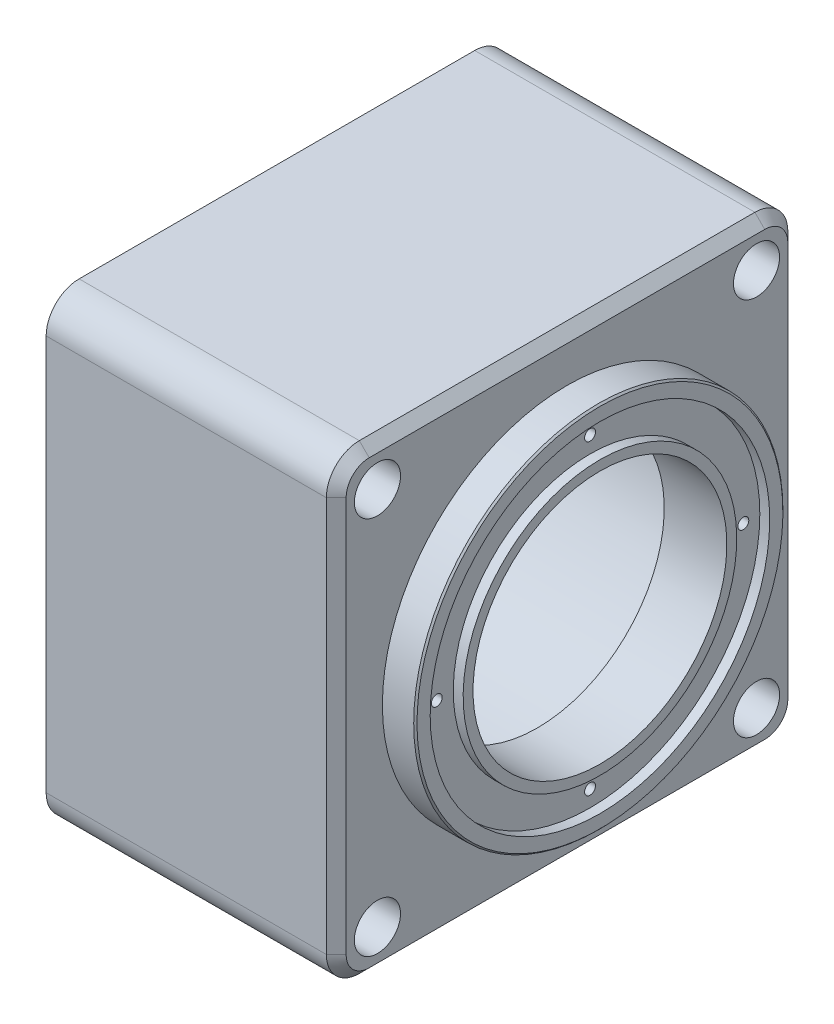
from build123d import *

# Parameters (mm, degrees)
SKETCH1_W               = 140
SKETCH1_H               = 140
BOSS_EXTRUDE1_DEPTH     = 88
SKETCH2_R               = 56
BOSS_EXTRUDE2_DEPTH     = 10
SKETCH3_R               = 60
CUT_EXTRUDE1_DEPTH      = 76
SKETCH4_R               = 38.5
CUT_EXTRUDE2_DEPTH      = 49
M10_TAPPED_HOLE1_D      = 8.5
M10_TAPPED_HOLE1_DEPTH  = 35
M10_TAPPED_HOLE1_TIP    = 2.553657631
M16_TAPPED_HOLE1_D      = 14
M16_TAPPED_HOLE1_DEPTH  = 35
M16_TAPPED_HOLE1_TIP    = 4.206024333
SKETCH14_R              = 55
CUT_EXTRUDE5_DEPTH      = 3
CHAMFER2_SIZE           = 0.5
BOSS_EXTRUDE3_START     = 44
SKETCH17_R              = 60
BOSS_EXTRUDE3_DEPTH     = 15
SKETCH18_R              = 55
CUT_EXTRUDE7_DEPTH      = 15
SKETCH22_R              = 60
CUT_EXTRUDE8_DEPTH      = 15
SKETCH23_R              = 51.5
SKETCH23_R_2            = 41.5
CUT_EXTRUDE9_DEPTH      = 3
CIRPATTERN1_COUNT       = 4
FILLET1_R               = 10
CHAMFER6_SIZE           = 3
SKETCH30_R              = 2.5
CUT_EXTRUDE12_DEPTH     = 12
G1_8_TAPPED_HOLE1_D     = 8.8
G1_8_TAPPED_HOLE1_DEPTH = 22.18
G1_8_TAPPED_HOLE1_TIP   = 2.643786724
SKETCH34_R              = 11
CUT_EXTRUDE14_DEPTH     = 3


with BuildPart() as part:
    # Sketch1 → Boss-Extrude1 (new body)
    with BuildSketch(Plane(origin=(0, 0, 0), x_dir=(0, -1, 0), z_dir=(1, 0, 0))):
        Rectangle(SKETCH1_W, SKETCH1_H)
    extrude(amount=BOSS_EXTRUDE1_DEPTH)

    # Sketch2 → Boss-Extrude2 (add)
    with BuildSketch(Plane(origin=(88, 0, 0), x_dir=(0, -1, 0), z_dir=(1, 0, 0))):
        with Locations(Location((0, 0, 0), (0, 0, 180))):
            Circle(SKETCH2_R)
    extrude(amount=BOSS_EXTRUDE2_DEPTH)

    # Sketch3 → Cut-Extrude1 (cut)
    with BuildSketch(Plane(origin=(0, 0, 0), x_dir=(0, -1, 0), z_dir=(-1, 0, 0))):
        Circle(SKETCH3_R)
    extrude(amount=-CUT_EXTRUDE1_DEPTH, mode=Mode.SUBTRACT)

    # Sketch4 → Cut-Extrude2 (cut)
    with BuildSketch(Plane(origin=(98, 0, 0), x_dir=(0, -1, 0), z_dir=(1, 0, 0))):
        with Locations(Location((0, 0, 0), (0, 0, 180))):
            Circle(SKETCH4_R)
    extrude(amount=-CUT_EXTRUDE2_DEPTH, mode=Mode.SUBTRACT)

    # M10 Tapped Hole1
    with Locations(Plane(origin=(0, 0, 0), x_dir=(0, 1, 0), z_dir=(-1, 0, 0))):
        with Locations((-35, 60), (35, 60), (60, 35), (60, -35), (35, -60), (-35, -60), (-60, -35), (-60, 35)):
            Hole(M10_TAPPED_HOLE1_D / 2, depth=M10_TAPPED_HOLE1_DEPTH)
            with Locations((0, 0, -(M10_TAPPED_HOLE1_DEPTH + M10_TAPPED_HOLE1_TIP / 2))):  # 118° drill point
                Cone(0, M10_TAPPED_HOLE1_D / 2, M10_TAPPED_HOLE1_TIP, mode=Mode.SUBTRACT)

    # M16 Tapped Hole1
    with Locations(Plane(origin=(88, 0, 0), x_dir=(0, -1, 0), z_dir=(1, 0, 0))):
        with Locations((57.5, 57.5), (-57.5, 57.5), (-57.5, -57.5), (57.5, -57.5)):
            Hole(M16_TAPPED_HOLE1_D / 2, depth=M16_TAPPED_HOLE1_DEPTH)
            with Locations((0, 0, -(M16_TAPPED_HOLE1_DEPTH + M16_TAPPED_HOLE1_TIP / 2))):  # 118° drill point
                Cone(0, M16_TAPPED_HOLE1_D / 2, M16_TAPPED_HOLE1_TIP, mode=Mode.SUBTRACT)

    # Sketch14 → Cut-Extrude5 (cut)
    with BuildSketch(Plane(origin=(76, 0, 0), x_dir=(0, -1, 0), z_dir=(-1, 0, 0))):
        Circle(SKETCH14_R)
    extrude(amount=-CUT_EXTRUDE5_DEPTH, mode=Mode.SUBTRACT)

    # Chamfer2
    chamfer2_edges = [part.edges().sort_by_distance(p)[0] for p in [
        (98, -56, 0),
    ]]
    chamfer(chamfer2_edges, length=CHAMFER2_SIZE)

    # Sketch17 → Boss-Extrude3 (add)
    with BuildSketch(Plane.ZY.offset(-76).offset(BOSS_EXTRUDE3_START)):
        with Locations(Location((0, 0, 0), (0, 0, 270))):
            Circle(SKETCH17_R)
    extrude(amount=-BOSS_EXTRUDE3_DEPTH)

    # Sketch18 → Cut-Extrude7 (cut)
    with BuildSketch(Plane.ZY.offset(-32)):
        with Locations(Location((0, 0, 0), (0, 0, 270))):
            Circle(SKETCH18_R)
    extrude(amount=-CUT_EXTRUDE7_DEPTH, mode=Mode.SUBTRACT)

    # Sketch22 → Cut-Extrude8 (cut)
    with BuildSketch(Plane.ZY.offset(-32)):
        with Locations(Location((0, 0, 0), (0, 0, 270))):
            Circle(SKETCH22_R)
    extrude(amount=-CUT_EXTRUDE8_DEPTH, mode=Mode.SUBTRACT)

    # Sketch23 → Cut-Extrude9 (cut)
    with BuildSketch(Plane(origin=(98, 0, 0), x_dir=(0, 0, -1), z_dir=(1, 0, 0))):
        with Locations(Location((0, 0, 0), (0, 0, 90))):
            Circle(SKETCH23_R)
        with Locations(Location((0, 0, 0), (0, 0, 90))):
            Circle(SKETCH23_R_2, mode=Mode.SUBTRACT)
    extrude(amount=-CUT_EXTRUDE9_DEPTH, mode=Mode.SUBTRACT)

    # Sketch25 → M4 Tapped Hole2 (revolve, cut)
    with BuildSketch(Plane(origin=(95, 46.5, 0), x_dir=(0, 0, -1), z_dir=(0, 1, 0))):
        Polygon((0, 0), (0, 11.091420021), (1.65, 10.1), (1.65, 0), align=None)
    m4_tapped_hole2 = revolve(axis=Axis((101.35, 46.5, 0), (-1, 0, 0)), mode=Mode.SUBTRACT)

    # CirPattern1: M4 Tapped Hole2 ×4 about axis
    cirpattern1_axis = Axis((0, 0, 0), (1, 0, 0))
    for i in range(1, CIRPATTERN1_COUNT):
        add(m4_tapped_hole2.rotate(cirpattern1_axis, i * 360 / CIRPATTERN1_COUNT), mode=Mode.SUBTRACT)

    # Fillet1
    fillet1_edges = [part.edges().sort_by_distance(p)[0] for p in [
        (44, -70, 70),
        (44, 70, 70),
        (44, 70, -70),
        (44, -70, -70),
    ]]
    fillet(fillet1_edges, radius=FILLET1_R)

    # Chamfer6
    chamfer6_edges = [part.edges().sort_by_distance(p)[0] for p in [
        (88, 0, -70),
        (88, -70, 0),
        (88, 70, 0),
        (88, 0, 70),
        (88, 67.071067812, 67.071067812),
        (88, 67.071067812, -67.071067812),
        (88, -67.071067812, 67.071067812),
        (88, -67.071067812, -67.071067812),
    ]]
    chamfer(chamfer6_edges, length=CHAMFER6_SIZE)

    # Sketch30 → Cut-Extrude12 (cut)
    with BuildSketch(Plane.XZ.offset(70)):
        with Locations(Location((43, 0, 0), (0, 0, 270))):
            Circle(SKETCH30_R)
    extrude(amount=-CUT_EXTRUDE12_DEPTH, mode=Mode.SUBTRACT)

    # G1/8 Tapped Hole1
    with Locations(Plane(origin=(0, -70, 0), x_dir=(-1, 0, 0), z_dir=(0, -1, 0))):
        with Locations((-43, 0)):
            Hole(G1_8_TAPPED_HOLE1_D / 2, depth=G1_8_TAPPED_HOLE1_DEPTH)
            with Locations((0, 0, -(G1_8_TAPPED_HOLE1_DEPTH + G1_8_TAPPED_HOLE1_TIP / 2))):  # 118° drill point
                Cone(0, G1_8_TAPPED_HOLE1_D / 2, G1_8_TAPPED_HOLE1_TIP, mode=Mode.SUBTRACT)

    # Sketch34 → Cut-Extrude14 (cut)
    with BuildSketch(Plane.XZ.offset(70)):
        with Locations(Location((43, 0, 0), (0, 0, 270))):
            Circle(SKETCH34_R)
    extrude(amount=-CUT_EXTRUDE14_DEPTH, mode=Mode.SUBTRACT)


solid = part.part
